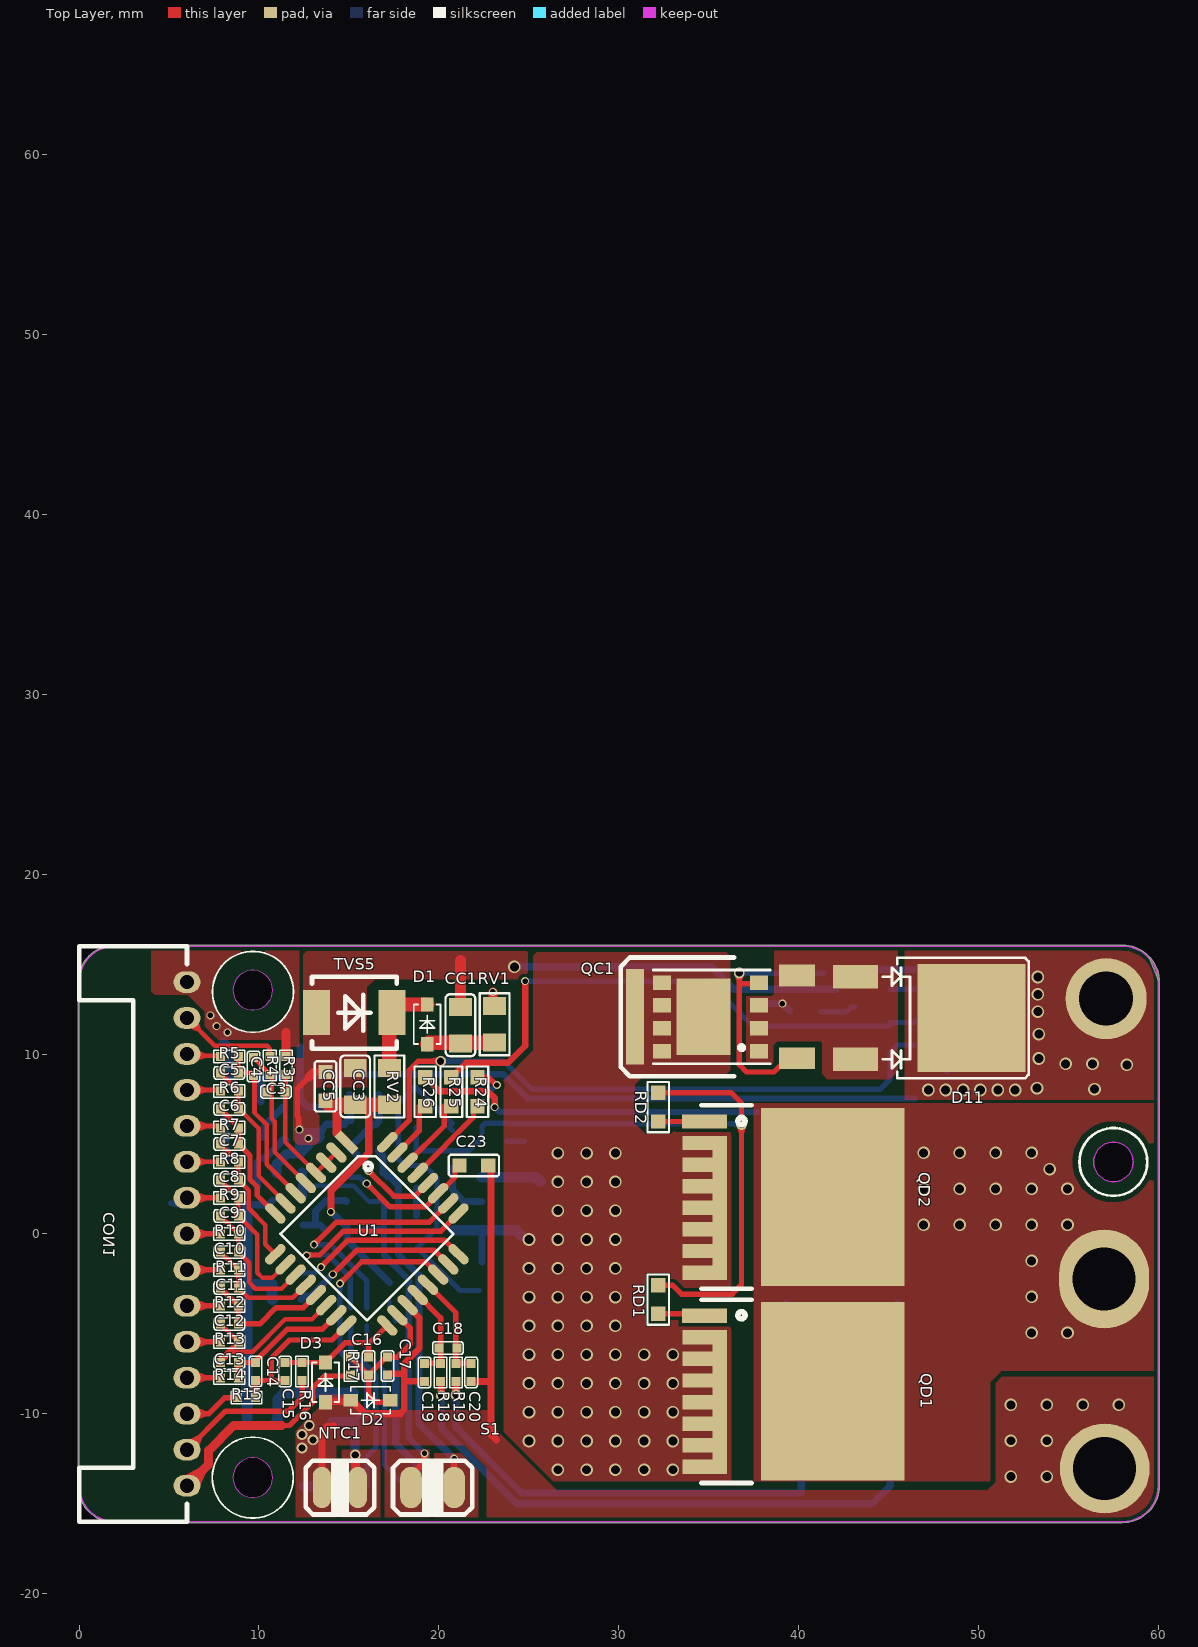
[diagram p0: Top Layer view]
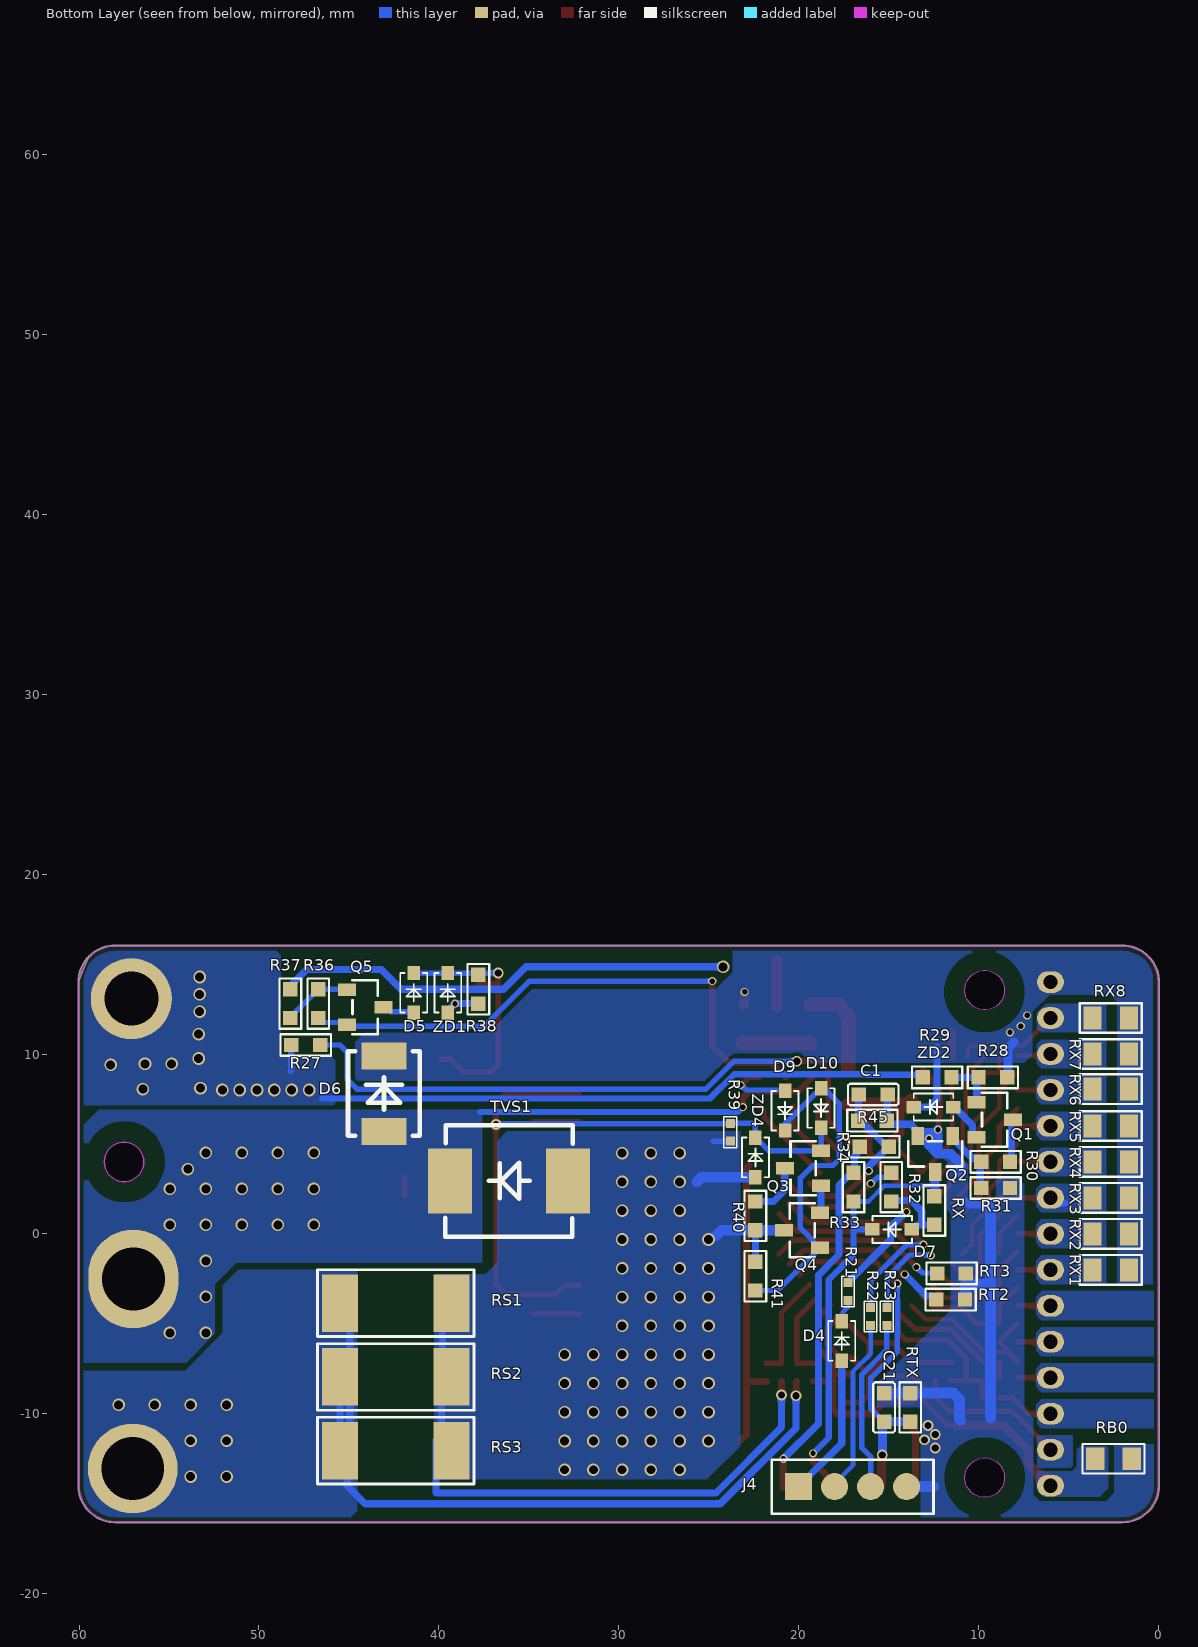
[diagram p1: Bottom Layer view, seen from below]
# Altium PCB MISC84412.PcbDoc
Units mm, origin at the board's own origin, x right, y up, seen from the top; angles counter-clockwise.
Board outline 60.1 x 32.1 mm, 2 copper layers (Top Layer, Bottom Layer); 110 components, 73 nets, 308 pads, 128 vias.

## Layer stack, top to bottom (the 12.6 mil dielectric is the usual default, probably not edited)
Top Solder: solder mask 0.0102, Solder Resist, Dk 3.5
Top Layer: signal copper 0.0356
Dielectric 1: dielectric 0.32, FR-4, Dk 4.8
Bottom Layer: signal copper 0.0356
Bottom Solder: solder mask 0.0102, Solder Resist, Dk 3.5

## Board outline
-0.05,-14.001 ccw(c2,-14) 2,-16.05 58,-16.05 ccw(c58,-14) 60.05,-14.001 60.05,14 60.05,-14 60.05,14 60.05,14.001 ccw(c58,14) 59.45,15.45 60.05,14.001 ccw(c58,14) 58,16.05 2,16.05 ccw(c2,14) -0.05,14
cut-out: 8.557,13.55 ccw(c9.657,13.55) 10.757,13.55 ccw(c9.657,13.55)
cut-out: 8.557,-13.55 ccw(c9.657,-13.55) 10.757,-13.55 ccw(c9.657,-13.55)
cut-out: 56.4,4 cw(c57.5,4) 58.6,4 cw(c57.5,4)

## Design rules (kind name [scope] priority, off if disabled: settings)
Clearance [All] p1: gap=0.2 ignorepadtopadclearanceinfootprint=FALSE
ComponentClearance [All] p1: gap=0 collisioncheckmode=3 verticalgap=0 showdistances=FALSE
HoleSize [All] p1: absolutevalues=TRUE maxlimit=50 minlimit=0.025 maxpercent=80.000 minpercent=20.000
HoleToHoleClearance [All] p1: gap=0 allowstackedmicrovias=TRUE
MinimumSolderMaskSliver [All] p1: minsoldermaskwidth=0
PlaneConnect [All] p1: planeconnectstyle=Direct reliefexpansion=0.508 reliefentries=4 reliefconductorwidth=0.254 reliefairgap=0.254
PolygonConnect [All] p1: connectstyle=Direct reliefconductorwidth=0.254 reliefentries=4 polygonreliefangle="90 Angle" airgapwidth=0.254
RoutingVias [All] p1: holewidth=0.4 width=0.6 viastyle="Through Hole" minholewidth=0.3 minwidth=0.45 maxholewidth=0.4 maxwidth=0.6
SilkToSilkClearance [All] p1: silktosilkclearance=0
SilkToSolderMaskClearance [IsPad] p1: minsilkscreentomaskgap=0 clearancetoexposedcopper=TRUE
SolderMaskExpansion [All] p1: expansion=0.102 istentingtop=FALSE
SupplyNets "Schematic Supply Nets_1" [InNet('B-')] p1: voltage=0.000
SupplyNets "Schematic Supply Nets" [InNet('VCC1')] p2: voltage=0.000
Width [All] p1: maxlimit=2 minlimit=0.254 preferedwidth=0.254 minimp=50.000000 maximp=50.000000 favimp=50.000000
23 further rules are at their usual default settings.

## Components (designator, comment, footprint, x,y, rotation, side; value= is the part's Value field where it differs from the comment)
C1 "0.1uF" C0603A 15.85,7.75 r180 bottom
C3 "0.1uF" C0402A 10.95,7.9 r0 top
C4 "0.1uF" C0402A 9.7,9.3 r90 top
C5 "0.1uF" C0402A 8.35,8.95 r0 top
C6 "0.1uF" C0402A 8.35,6.95 r0 top
C7 "0.1uF" C0402A 8.35,5 r0 top
C8 "0.1uF" C0402A 8.35,3 r0 top
C9 "0.1uF" C0402A 8.35,1 r0 top
C10 "0.1uF" C0402A 8.35,-1 r0 top
C11 "0.1uF" C0402A 8.35,-3 r0 top
C12 "0.1uF" C0402A 8.35,-5 r0 top
C13 "0.1uF" C0402A 8.35,-7.15 r180 top
C14 "0.1uF" C0402A 9.8,-7.65 r90 top
C15 "0.1uF" C0402A 11.45,-7.65 r270 top
C16 "0.1uF" C0402A 16.1,-7.35 r90 top
C17 "1uF" C0402A 17.15,-7.35 r90 top
C18 "1000PF" C0402A 20.5,-6.35 r180 top
C19 "1uF" C0402A 19.2,-7.7 r270 top
C20 "1uF" C0402A 21.8,-7.7 r270 top
C21 "1000PF" C0603A 15.25,-9.65 r90 bottom
C23 "1uF/25V" C0603A 21.95,3.8 r180 top
CC1 "1uF/100V" C0805L 21.2,11.6 r270 top
CC3 "1uF/100V" C0805L 15.35,8.2 r270 top
CC5 "100nF/100V" C0603A 13.7,8.2 r270 top
CON1 "Header 15" PH-2.0mm15P弯脚不带扣 6,0 r90 top locked
D1 "BAV21W" SOD323(1+2-) 19.35,11.65 r270 top
D2 "BAT46WS" SOD323(1+2-) 16.2,-9.25 r180 top
D3 "BAT46WS" SOD323(1+2-) 13.7,-8.25 r270 top
D4 "BAV21WS" SOD323(1+2-) 17.6,-5.95 r270 bottom
D5 "BAV21WS" SOD323(1+2-) 41.4,13.4 r270 bottom
D6 "RS3M" "SMB M(1+2-)" 43.05,7.8 r270 bottom
D7 "1N4148SW" SOD323 14.8,0.25 r180 bottom
D9 "BAV21WS" SOD323(1+2-) 20.75,6.85 r90 bottom
D10 "BAV21WS" SOD323(1+2-) 18.75,7 r90 bottom
D11 "MBR10100DCT" TO-252-DIODE-DUAL 46.387,12 r270 top
J4 "UART" CH-2.0-4P 17,-14.05 r180 bottom
NTC1 "10KNTC" RT2.3X1-2 14.5,-14.1 r180 top (schematic designator NC1)
Q1 "MMBT5401" SOT23-3_BEC 9.1,6.35 r270 bottom
Q2 "MMBT5551" SOT23-3_BEC 12.4,4.45 r0 bottom
Q3 "MMBT5401" SOT23-3 19.75,3.65 r90 bottom
Q4 "MMBT5401" SOT23-3 19.8,0.2 r90 bottom
Q5 "MMBT5401" SOT23-3 44.1,12.6 r270 bottom
QC1 "NMOS" TO-252-DFN 35.416,12.065 r0 top
QD1 "NMOS" TOLL 38.4,-8.75 r270 top value=60V75A@0.94
QD2 "NMOS" TOLL 38.4,2.05 r270 top value=60V75A@0.94
R3 "510R" R0402A 11.5,9.35 r90 top
R4 "510R" R0402A 10.6,9.35 r90 top
R5 "510R" R0402A 8.35,9.85 r180 top
R6 "510R" R0402A 8.35,7.95 r180 top
R7 "510R" R0402A 8.35,5.9 r180 top
R8 "510R" R0402A 8.35,4 r180 top
R9 "510R" R0402A 8.35,2 r180 top
R10 "510R" R0402A 8.35,0 r180 top
R11 "510R" R0402A 8.35,-2 r180 top
R12 "510R" R0402A 8.35,-4 r180 top
R13 "510R" R0402A 8.35,-6 r180 top
R14 "510R" R0402A 8.35,-8 r180 top
R15 "510R" R0402A 9.3,-9.1 r0 top
R16 "510R" R0402A 12.4,-7.65 r270 top
R17 "510R" R0402A 15.1,-7.35 r270 top
R18 "10R" R0402A 20.1,-7.7 r270 top
R19 "10R" R0402A 20.95,-7.7 r270 top
R21 "100R" R0402A 17.25,-3.2 r90 bottom
R22 "100R" R0402A 16,-4.6 r90 bottom
R23 "100R" R0402A 15.1,-4.6 r90 bottom
R24 "1K" R0603A#1 22.15,7.9 r270 top
R25 "1K" R0603A#1 20.7,7.9 r270 top
R26 "1M" R0603A#1 19.25,7.9 r270 top
R27 "3M" R0603A#2 47.4,10.5 r180 bottom
R28 "20K" R0603A#2 9.2,8.7 r180 bottom
R29 "100K" R0603A#2 12.3,8.7 r180 bottom
R30 "1M" R0603A#2 9.05,4 r180 bottom
R31 "100K" R0603A#2 9.05,2.55 r0 bottom
R32 "100K" R0603A#2 14.85,2.6 r270 bottom
R33 "0Ω/NC" R0603A#2 16.95,2.6 r270 bottom
R34 "100K" R0603A#2 15.8,4.85 r180 bottom
R36 "1M" R0603A#2 46.7,12.8 r270 bottom
R37 "3M" R0603A#2 48.25,12.8 r90 bottom
R38 "1M" R0603A#2 37.8,13.6 r90 bottom
R39 "10M" R0402A 23.8,5.65 r90 bottom
R40 "510R" R0603A#2 22.4,1 r270 bottom
R41 "4.7M" R0603A#2 22.4,-2.35 r270 bottom
R45 "10M" R0603A#2 15.9,6.3 r180 bottom
RB0 "51R" R0805L 2.5,-12.5 r0 bottom
RD1 "47R" R0603Ap 32.2,-3.65 r270 top
RD2 "47R" R0603Ap 32.2,7.05 r270 top
RS1 "R005" R2512L 42.4,-3.85 r180 bottom
RS2 "R005" R2512L 42.4,-7.95 r180 bottom
RS3 "R005" R2512L 42.4,-12.05 r180 bottom
RT2 "10K" R0603A#2 11.55,-3.65 r180 bottom
RT3 "10K" R0603A#2 11.5,-2.2 r180 bottom
RTX "NC" R0603A#2 13.8,-9.65 r90 bottom
RV1 "1KΩ" R0805L 23.1,11.65 r90 top
RV2 "100Ω" R0805L 17.25,8.2 r90 top
RX "0R" R0603A#2 12.45,1.3 r270 bottom
RX1 "0Ω" R0805L 2.65,-2 r0 bottom
RX2 "0Ω" R0805L 2.65,0 r0 bottom
RX3 "0Ω" R0805L 2.65,2 r0 bottom
RX4 "0Ω" R0805L 2.65,4 r0 bottom
RX5 "0Ω" R0805L 2.65,6 r0 bottom
RX6 "0Ω" R0805L 2.65,8.05 r0 bottom
RX7 "0Ω" R0805L 2.65,10 r0 bottom
RX8 "0Ω" R0805L 2.65,12 r0 bottom
S1 "SW-SPST" RT2.3X1.2-2 19.65,-14.1 r0 top
TVS1 "75CA" SMC 36.1,2.95 r0 bottom
TVS5 "SMBJ64A" "SMB M(1+2-)" 15.3,12.3 r180 top
U1 "SH3676016B" LQFP32L(PIN间距0.8mm) 16,0 r315 top
ZD1 "15V" SOD323(1+2-) 39.5,13.4 r270 bottom
ZD2 "15V" SOD323(1+2-) 12.5,7.05 r180 bottom
ZD4 "15V" SOD323(1+2-) 22.4,4.25 r270 bottom

## Footprints (in the part's own frame and the unit in brackets; to place one, negate y for a bottom-side part, rotate by r counter-clockwise, add the part's x,y. Pads: shape width x height; smd on the part's side, far side on the other; paste and mask are expansions set on the pad)
C0402A [mm] "贴片电容"
  rect 0.5x0.5 smd paste+0 mask+0.05: 1(-0.5,0) 2(0.5,0)
  silkscreen extent -0.85,-0.35 0.85,0.35
C0603A [mm] "贴片电容"
  rect 0.8x0.8 smd mask+0.08: 1(-0.8,0) 2(0.8,0)
  silkscreen extent -1.4,-0.6 1.4,0.6
C0805L [mil] "贴片电容"
  rect 40x50 smd paste+0 mask+1.97: 1(-40,0) 2(40,0)
  silkscreen extent -68,-32 68,32
CH-2.0-4P [mm] "测试座2.0mm"
  rect 1.5x1.5 smd: 1(-3,0)
  round 1.5 smd: 2(-1,0) 3(1,0) 4(3,0)
  silkscreen extent -4.5,-1.5 4.5,1.5
LQFP32L(PIN间距0.8mm) [mm] "贴片IC(中颖SH3676014/16BP)"
  rect 1.4x0.5 smd: 1(-4.4,2.8)
  oval 1.4x0.5 smd: 2(-4.4,2) 3(-4.4,1.2) 4(-4.4,0.4) 5(-4.4,-0.4) 6(-4.4,-1.2) 7(-4.4,-2) 8(-4.4,-2.8) 17(4.4,-2.8) 18(4.4,-2) 19(4.4,-1.2) 20(4.4,-0.4) 21(4.4,0.4) 22(4.4,1.2) 23(4.4,2) 24(4.4,2.8)
  oval 0.5x1.4 smd: 9(-2.8,-4.4) 10(-2,-4.4) 11(-1.2,-4.4) 12(-0.4,-4.4) 13(0.4,-4.4) 14(1.2,-4.4) 15(2,-4.4) 16(2.8,-4.4) 25(2.8,4.4) 26(2,4.4) 27(1.2,4.4) 28(0.4,4.4) 29(-0.4,4.4) 30(-1.2,4.4) 31(-2,4.4) 32(-2.8,4.4)
  silkscreen extent -3.4,-3.4 3.4,3.4
PH-2.0mm15P弯脚不带扣 [mm] "PH-2.0mm15P弯脚不带扣连接器"
  oval 1.2x1.5 hole 0.8: 1(-14,0) 2(-12,0) 3(-10,0) 4(-8,0) 5(-6,0) 6(-4,0) 7(-2,0) 8(0,0) 9(2,0) 10(4,0) 11(6,0) 12(8,0) 13(10,0) 14(12,0) 15(14,0)
  silkscreen extent -16,0 16,6
R0402A [mm] "贴片电阻"
  rect 0.5x0.5 smd paste+0 mask+0.05: 1(-0.5,0) 2(0.5,0)
  silkscreen extent -0.85,-0.35 0.85,0.35
R0603A#1 [mm] "贴片电阻"
  rect 0.8x0.8 smd mask+0.08: 1(-0.8,0) 2(0.8,0)
  silkscreen extent -1.4,-0.6 1.4,0.6
R0603A#2 [mm] "贴片电阻"
  rect 0.8x0.8 smd mask+0.102: 1(-0.8,0)
  rect 0.8x0.8 smd mask+0.08: 2(0.8,0)
  silkscreen extent -1.4,-0.6 1.4,0.6
R0603Ap [mm] "贴片电阻"
  rect 0.8x0.8 smd mask+0.08: 1(-0.8,0) 2(0.8,0)
  Top Layer pour cut-out: -1.5,0.7 1.5,0.7 1.5,-0.7 -1.5,-0.7
  silkscreen extent -1.4,-0.6 1.4,0.6
R0805L [mil] "贴片电阻"
  rect 40x50 smd paste+0 mask+1.97: 1(-40,0) 2(40,0)
  silkscreen extent -68,-32 68,32
R2512L [mm] "贴片电阻"
  rect 2x3.2 smd: 1(-3.1,0) 2(3.1,0)
  silkscreen extent -4.35,-1.85 4.35,1.85
RT2.3X1-2 [mm] "焊线NTC"
  oval 1x2.3 smd: 1(-1,0) 2(1,0)
  silkscreen extent -1.9,-1.55 1.9,1.5
RT2.3X1.2-2 [mm] "焊线NTC"
  oval 1.2x2.3 smd: 1(-1.2,0) 2(1.2,0)
  silkscreen extent -2.2,-1.55 2.2,1.5
"SMB M(1+2-)" [mm] "贴片二极管"
  rect 1.5x2.5 smd: 1(2.1,0) 2(-2.1,0)
  silkscreen extent -2.35,-2 2.35,2
SMC [mm]
  rect 2.44x3.62 smd: 1(-3.275,0) 2(3.275,0)
  silkscreen extent -3.55,-3.1 3.55,3.1
SOD323 [mm] "贴片二极管"
  rect 0.8x0.7 smd: 1(-1.1,0) 2(1.1,0)
  silkscreen extent -1.1,-0.75 1.1,0.75
SOD323(1+2-) [mm] "贴片二极管"
  rect 0.8x0.7 smd: 1(1.1,0) 2(-1.1,0)
  silkscreen extent -1.1,-0.75 1.1,0.75
SOT23-3 [mm] "贴片IC/MOS*"
  rect 0.7x1 smd: 1(-0.975,-1) 2(0.975,-1) 3(0,1.016)
  silkscreen extent -1.5,-0.7 1.5,0.7
SOT23-3_BEC [mm] "贴片IC/MOS*"
  rect 0.7x1 smd: B(-0.975,-1) C(0,1.016) E(0.975,-1)
  silkscreen extent -1.5,-0.7 1.5,0.7
TO-252-DFN [mm]
  rect 1x0.8 smd: 1(2.384,1.905) 2(2.384,-1.905) 2(2.384,-0.635) 2(2.384,0.635) 3(-3.016,-1.905) 3(-3.016,-0.635) 3(-3.016,0.635) 3(-3.016,1.905)
  rect 2x1.2 smd: 1(4.5,-2.3) 2(4.5,2.3)
  rect 1x5.3 smd: 3(-4.5,0)
  rect 3x4.26 smd: 3(-0.716,0)
  silkscreen extent -5.31,-3.3 3,3.3
TO-252-DIODE-DUAL [mm] "贴片二极管"
  rect 1.3x2.5 smd: 1(-2.3,-3.212) 2(2.3,-3.212)
  rect 6x6 smd: 3(0,3.213)
  silkscreen extent -3.35,-1.7 3.35,6.4
TOLL [mm] "贴片MOS"
  rect 0.8x2.5 smd: 1(-4.2,-3.638)
  rect 0.8x1.7 smd: 2(-3,-4) 2(-1.8,-4) 2(-0.6,-4) 2(0.6,-4) 2(1.8,-4) 2(3,-4) 2(4.2,-4)
  rect 8x0.8 smd: 2(0.6,-2.788)
  rect 9.9x8 smd: 3(0,3.5)
  silkscreen extent -5.1,-3.8 5.1,-1

## Part data
C1 C23: library part CAP, "CAP"
C3 C4 C5 C6 C7 C8 C9 C10 C11 C12 C13 C14 C15 C16 C17 C18 C19 C20 C21 CC1 CC3 CC5: library part "0805 100nF(104) 10% 50V", "SMD capacitor", Package=0805, SuppliersPartNumber=C49678
CON1: "Header15"
D1: library part "SOD-323 1N4148WS T4", "Diode", Package=SOD-323, SuppliersPartNumber=C2128
D2 D3 D4 D5 D6 D9 D10: library part DIODE, "DIODE"
D7: "SMD diode"
D11: "SMD dual diode, common cathode"
J4: library part CON4
NTC1 RT2 RT3: library part RES2, "RES"
Q1: library part PNP, "PNP Transistor"
Q2: library part NPN, "NPN Transistor"
Q3 Q4 Q5: library part 8550, "PNP"
QC1: library part MOSFET-N
QD1 QD2: library part IRFR014, "HEXFET N-Channel Power MOSFET"
R3 R4 R5 R6 R7 R8 R9 R10 R11 R12 R13 R14 R15 R16 R17 R18 R19 RS1 RS2 RS3: library part "0603 1KΩ (1001) 1%", "SMD resistor", Package=0603, SuppliersPartNumber=C21190
R21 R22 R23 R24 R25 R26 R27 R28 R29 R30 R31 R32 R33 R34 R36 R37 R38 R39 R40 R41 R45 RTX RX: library part RES1, "RES"
RB0: library part RES1, "±5% /UniOhm/yageo/TA-I/Walsin/Ralec"
RD1 RD2: library part "0603 1.2MΩ (1204) 1%", "SMD resistor", Package=0603, SuppliersPartNumber=C22766
RV1 RV2 RX1 RX2 RX3 RX4 RX5 RX6 RX7 RX8: library part "0805 300Ω (3000) 1%", "SMD resistor", Package=0805, SuppliersPartNumber=C17617
S1: "Single-Pole, Single-Throw Switch"
TVS1: library part TVS, "TVS"
TVS5: library part "LL-34 ZMM5V6", "Zener diode", Package=LL-34, SuppliersPartNumber=C8062
ZD1 ZD2 ZD4: library part ZENOR, "ZENOR"

## Free pads (board coordinates)
  round 0.025 on Keep-Out: 1(52.327,65.458) 1(56.137,-19.886)
  rect 2.5x15 on Bottom Solder: 2(25.9,-3.65) 2(29.039,-3.638)
  rect 2.5x15 on Top Solder: 2(26.3,-4.85) 2(29.3,-4.85)
  rect 2.5x20 on Top Solder: 2(48.7,-3.35)
  rect 2.5x12 on Top Solder: 2(51.789,0.262)
  oval 5x5.5 hole 3.5: 2(56.986,-2.51)
  round 5 hole 3.5: 2(57.017,-13.049)
  round 4.5 hole 3: 2(57.098,13.075)

## Via types
v1: diameter 0.7, hole 0.5, Top Layer to Bottom Layer, tented both sides, 98 vias
v2: diameter 0.45, hole 0.3, Top Layer to Bottom Layer, tented both sides, 20 vias
v3: diameter 0.6, hole 0.4, Top Layer to Bottom Layer, tented both sides, 10 vias

## Nets (pads, with @x,y where several pads share a name; then routed paths per layer and width w, separated by ;. In a path a pad name is that pad's centre, name@x,y a point inside that pad or via, vN(x,y) a via of type N, cw(c..) or ccw(c..) an arc to the next point about the centre after c; other vN are vias at no path point)
B0: CON1.1 R17.2 RB0.2 | length 12.6
  Top Layer w0.3: 11.25,-10.65 11.7,-10.65 12.55,-9.8 13,-9.35 13,-8.55 13.65,-7.9 15.1,-7.9 R17.2
  Top Layer w0.5: CON1.1 7.2,-12.8 7.2,-12.05 8.6,-10.65 11.25,-10.65
B1: CON1.2 R16.2 | length 8.6
  Top Layer w0.3: CON1.2 8.15,-9.85 11.65,-9.85 12.4,-9.1 R16.2
B2: CON1.3 R15.1 | length 3.2
  Top Layer w0.3: CON1.3 7.2,-10 8.1,-9.1 R15.1
B3: CON1.4 R14.2 | length 1.9
  Top Layer w0.3: CON1.4 R14.2
B4: CON1.5 R13.2 | length 2
  Top Layer w0.3: CON1.5@6.1,-5.9 CON1.5 R13.2
B5: CON1.6 R12.2 | length 2.1
  Top Layer w0.3: CON1.6@6.2,-4.2 CON1.6 R12.2
B6: CON1.7 R11.2 RX1.2 | length 1.9
  Top Layer w0.3: CON1.7 R11.2
B7: CON1.8 R10.2 RX2.2 | length 1.9
  Top Layer w0.3: CON1.8 R10.2
B8: CON1.9 R9.2 RX3.2 | length 2.8
  Top Layer w0.3: CON1.9 R9.2@7.8,2
  Bottom Layer w0.3: 5.1,1.7 CON1.9@6,1.7 ; CON1.9 CON1.9@6.1,1.9
B9: CON1.10 R8.2 RX4.2 | length 1.9
  Top Layer w0.254: CON1.10 R8.2
B10: CON1.11 R7.2 RX5.2 | length 1.9
  Top Layer w0.3: CON1.11 R7.2@7.85,6
B11: CON1.12 R6.2 RX6.2 | length 2.3
  Top Layer w0.254: CON1.12@6.34,7.66 CON1.12 R6.2@7.85,8
B12: CON1.13 R5.2 RX7.2 | length 1.9
  Top Layer w0.254: CON1.13 6.1,9.9 R5.2@7.85,9.9
B13: CON1.14 R4.2 RX8.2 | length 5.8
  Top Layer w0.254: CON1.14 7.55,10.45 10.451,10.45 10.6,10.301 R4.2
B+: CON1.15 D6.2 R3.2 R28.2 RV1.2 RX1.1 RX2.1 RX3.1 RX4.1 RX5.1 RX6.1 RX7.1 RX8.1 ZD2.2 | length 8.8
  Top Layer w0.5: R3.2 11.5,11.191 ; v2(23,13.45) 23,12.766 RV1.2
  Bottom Layer w0.4: 12.3,10.375 12.3,7.484 12.734,7.05 ZD2.2
  Bottom Layer w0.5: 8.035,10.665 8.35,10.35 R28.2@8.35,8.55
  other v2: 8.25,11.2 7.65,11.55 7.3,12.15
B-: C1.2 C17.1 C19.2 C20.2 C21.2 C23.1 CC1.1 CC3.1 CC5.1 D2.1 D3.1 J4.4 NTC1.2 pad.2@57.017,-13.049 Q2.E R18.2 R31.1 R37.2 R45.2 RB0.1 RS1.1 RS2.1 RS3.1 RT2.2 RT3.2 RTX.2 TVS5.1 U1.19 | length 143.1
  Top Layer w0.3: v2(12.25,5.8) 12.221,5.829 12.221,6.459 12.125,6.555 12.125,8.06 12.791,8.726
  Top Layer w0.35: C17.1 17.225,-7.775 18.05,-7.775 18.075,-7.8 18.075,-8.1 ; 17.866,-10 17.916,-9.95 17.916,-9.915 18.075,-9.755 18.075,-8.1 ; 18.075,-7.775 18.075,-7.204 18.925,-6.354 18.925,-4.663 18.263,-4 U1.19 ; C19.2 18.175,-8.2 18.075,-8.1 ; R18.2 20.125,-8.225 v3@20.125,-8.975
  Top Layer w0.4: 13.075,9.01 13.1,9.01 ; NTC1.2 13.5,-11 13.812,-10.688 14.112,-10.688 14.15,-10.65 ; D3.1 13.75,-9.3 D2.1@15.1,-9.3 ; D2.1 15.15,-9.25 15.9,-10 17.866,-10 ; C20.2 22.85,-8.2 22.9,-8.15 ; C23.1 22.9,3.65 22.9,-8.15 ; 23.2,-11.45 22.9,-11.15 22.9,-8.15
  Top Layer w0.5: 12.791,8.726 13.075,9.01
  Top Layer w0.6: CC1.1 21.2,15.2
  Bottom Layer w0.4: 9.331,1.469 9.331,1.619 10.516,1.619 10.75,1.853 ; v2(12.25,5.8) 12.267,5.783 12.434,5.616 v2@12.6,5.45 ; Q2.E@13.362,5.713 13.487,5.713 13.525,5.75 13.525,5.862 13.759,6.096 14.746,6.096 R45.2@14.95,6.3 ; C1.2 15.075,7.725 15.075,6.325 R45.2 ; v3(20.15,-9) 20.15,-10.8 24.35,-15 44.112,-15 45.097,-14.016 45.097,-12.653 RS3.1@45.5,-12.25 ; v1(24.2,14.85) 35.15,14.85 36.4,13.6 42.1,13.6 43.2,14.7 47.35,14.7 R37.2@48.25,13.8 ; RS2.1@45.5,-8.05 RS3.1 RS3.1@45.5,-12.25 ; RS1.1 44.95,-4.4 44.95,-7.95 44.95,-12.25 RS3.1@45.5,-12.25
  Bottom Layer w0.55: 10.966,3.389 10.966,3.871 11.548,4.452 12.267,4.452 ; v2@12.267,5.783 12.267,4.452 ; 12.434,5.616 13.3,5.616 13.375,5.541 Q2.E 13.375,5.375 13.3,5.3 v2(12.75,5.3) 12.75,4.935 12.267,4.452
  Bottom Layer w0.6: 9.331,-10.237 9.331,1.469 ; 9.406,-2.8 10.725,-2.8 10.725,-3.625 RT2.2 ; 11,-10.35 11.05,-10.3 11.05,-9.201 11.401,-8.85 RTX.2 C21.2 ; 12.5,-14.05 J4.4 ; C21.2@15.244,-8.844 C21.2@15.25,-8.837
  other v1: 51.8,-13.5 53.8,-13.5 51.8,-11.5 53.8,-11.5 51.8,-9.5 53.8,-9.5 55.8,-9.5 57.8,-9.5
  other v3: 12.4,-11.9 13,-11.45 12.4,-11.15 12.8,-10.65
C-: D11.3 pad.2@57.098,13.075 R27.1 R29.1 | length 35.5
  Bottom Layer w0.35: R29.1 13.25,8.85 16.2,8.85 16.225,8.875 23.583,8.875 24.933,7.525 46.475,7.525 ; R27.1 48.2,9.1 48.25,9.05
  other v1: 47.214,8 48.179,8 49.143,8 50.107,8 51.071,8 52.036,8 56.45,8.05 53.25,8.1 58.25,9.4 54.85,9.45 56.336,9.45 53.35,9.75 53.35,11.1 53.3,12.35 53.3,13.314 53.3,14.279
CHG1: Q5.2 R25.1 R36.2 | length 31.5
  Top Layer w0.35: R25.1 21.512,9.513 23.862,9.513 24.8,10.45 v2(24.8,14.05)
  Bottom Layer w0.3: v2(24.8,14.05) 34.95,14.05 37.45,11.55 45.025,11.55 Q5.2 ; Q5.2@45.1,11.75 46.45,11.75 R36.2
CTLD: C1.1 R34.2 R45.1 U1.28 | length 9.4
  Top Layer w0.3: v2(16.1,3.5) 17.5,2.1 18.666,2.1 U1.28
  Bottom Layer w0.4: R34.2 16.09,3.76 16.09,3.51 v2(16.1,3.5) ; R34.2@15.25,5 16.35,6.1 16.5,6.1 16.675,6.275 16.675,7.725 C1.1
DSG1: D9.1 R24.1 | length 3.9
  Top Layer w0.3: R24.1 22.759,8.7 23.184,8.275 v2(23.225,8.275)
  Bottom Layer w0.3: D9.1 20.8,8 22.909,8 23.184,8.275 v2(23.225,8.275)
NetC18_1: C18.1 C20.1 R19.1 U1.21 | length 5.9
  Top Layer w0.3: U1.21 20.95,-4.384 R19.1 C20.1
NetC18_2: C18.2 C19.1 R18.1 U1.20 | length 5.2
  Top Layer w0.3: U1.20 20.1,-4.666 R18.1 C19.1
NetC21_1: C21.1 NTC1.1 RTX.1 U1.22 | length 19.8
  Top Layer w0.3: v2(14.507,-2.757) 15.714,-1.55 19.247,-1.55 U1.22
  Top Layer w0.5: v3(15.35,-12.3) 15.369,-12.319 15.369,-12.966 15.404,-13.001 15.404,-14.004 NTC1.1
  Bottom Layer w0.3: v2(14.507,-2.757) 14.507,-3.698 14.5,-3.705 14.5,-5.495 14.507,-5.502 14.507,-6.551 16,-8.044 16,-9.7 15.331,-10.369 C21.1@15.331,-10.6
  Bottom Layer w0.5: RTX.1@14.05,-10.45 14.063,-10.438 C21.1@15.25,-10.438 ; C21.1@15.331,-10.6 15.331,-12.281 v3(15.35,-12.3)
NetCC1_2: CC1.2 D1.1 RV1.1 | length 3.8
  Top Layer w0.8: D1.1 19.434,10.634 RV1.1
NetD1_2: D1.2 RV2.2 TVS5.2 | length 4.9
  Top Layer w0.8: RV2.2@17.25,9.108 17.25,12.15 TVS5.2 ; TVS5.2@17.75,12.75 D1.2
NetD4_1: D4.1 J4.1 | length 8
  Bottom Layer w0.4: D4.1 17.6,-11.65 J4.1
NetD4_2: D4.2 R21.1 | length 1.3
  Bottom Layer w0.254: R21.1 17.25,-4.05 17.55,-4.35 17.55,-4.8 D4.2
NetD5_1: D5.1 Q5.3 | length 1.9
  Bottom Layer w0.3: D5.1@41.25,12.35 42.684,12.35 42.934,12.6 Q5.3
NetD5_2: D5.2 QC1.1 R38.2 ZD1.2 | length 14.6
  Top Layer w0.3: v3(36.7,14.5) 36.7,13.9 ; QC1.1@37.8,13.905 36.705,13.905 36.7,13.9 ; QC1.1@39.916,9.7 39.327,9.7 38.627,9 37.104,9 36.7,9.404 36.7,13.9
  Bottom Layer w0.3: v3(36.7,14.5) R38.2@37.8,14.5 ; R38.2 37.9,14.5 ZD1.2 D5.2
NetD7_1: D7.1 Q2.C R33.2 RX.1 S1.1 | length 24.4
  Top Layer w0.35: S1.1 18.45,-13.421 19.181,-12.69 19.181,-12.219 v2(19.2,-12.2)
  Bottom Layer w0.254: 12.425,2.7 12.452,2.673 15.239,2.673 16.112,1.8 R33.2
  Bottom Layer w0.35: D7.1 16.85,0.25 16.95,0.15 ; R33.2@16.95,1.75 16.95,0.15 ; v2@19.187,-12.187 18.325,-11.325 18.325,-2.55 16.95,-1.175 16.95,0.15
  Bottom Layer w0.5: Q2.C 12.425,3.409 12.425,2.7 12.425,2.125 RX.1
NetD7_2: D7.2 R32.2 RX.2 | length 4.1
  Bottom Layer w0.4: RX.2 13.05,0.5 ; D7.2 13.65,0.25 13.4,0.5 13.05,0.5 ; R32.2 14.8,1.85 13.741,1.85 13.15,1.259 13.15,0.6 13.05,0.5
NetD9_2: D9.2 D10.1 Q4.1 R41.2 | length 18.8
  Bottom Layer w0.3: D10.1@18.675,8.175 17.75,7.25 17.75,4.15 18.1,3.8 19.2,3.8 19.9,3.1 19.9,0.325 Q4.1 21.175,-3.15 R41.2@22.25,-3.15 ; D10.1 20.557,6.293 20.7,6.15 20.75,6.15 ; D9.2@20.582,5.918 D9.2
NetD10_2: D10.2 Q3.2 R39.2 RD1.1 RD2.1 ZD4.2 | length 40.4
  Top Layer w0.3: RD1.1 33,-2.85 33.5,-3.35 36.3,-3.35 36.825,-2.825 v3(36.825,6.075) 36.825,7.275 36.25,7.85 RD2.1
  Bottom Layer w0.3: D10.2 Q3.2 21.675,4.625 22.15,5.1 22.2,5.1 22.4,5.3 ZD4.2 22.4,5.974 22.576,6.15 R39.2 23.838,6.112 31.917,6.112 36.788,6.112 v3(36.825,6.075)
NetD11_1: D11.1 D11.2 QC1.2 R38.1 ZD1.1 | length 1.9
  Bottom Layer w0.4: R38.1 v2(39.1,12.8) ZD1.1@39.5,12.4
NetJ4_2: J4.2 R22.1 | length 9.8
  Bottom Layer w0.254: R22.1 16,-6.662 16.977,-7.639 16.977,-12.855 18,-13.878 J4.2
NetJ4_3: J4.3 R23.1 | length 9.7
  Bottom Layer w0.3: R23.1 15.1,-6.437 16.5,-7.837 16.5,-11.888 16,-12.388 J4.3
NetQ1_B: Q1.B R28.1 R29.2 | length 2.8
  Bottom Layer w0.4: R28.1 R29.2 ; Q1.B R28.1@10.1,8.65
NetQ1_C: Q1.C R30.2 | length 2.4
  Bottom Layer w0.4: Q1.C 8.167,6.267 8.167,4.083 R30.2
NetQ1_E: Q1.E ZD2.1 | length 2.3
  Bottom Layer w0.4: Q1.E 10.187,5.375 10.337,5.525 10.337,6.037 11.35,7.05 ZD2.1
NetQ2_B: Q2.B R30.1 R31.2 | length 3.2
  Bottom Layer w0.4: R31.2@9.9,2.65 9.9,3.55 9.9,3.75 R30.1@9.9,3.95 ; R30.1@10.05,4.2 10.341,4.2 11,4.859 11,4.875 11.325,5.2 Q2.B@11.5,5.2
NetQ3_1: Q3.1 Q4.2 | length 1.5
  Bottom Layer w0.4: Q4.2@18.75,1.025 Q3.1@18.75,2.535
NetQ3_3: Q3.3 R40.1 | length 3.1
  Bottom Layer w0.4: Q3.3 20.766,2.434 21.4,1.8 R40.1
NetQ5_1: Q5.1 R36.1 R37.1 | length 3.9
  Bottom Layer w0.3: Q5.1 45.125,13.6 R36.1 48,12.3 48,12.25 R37.1
NetQD1_1: QD1.1 RD1.2 | length 2.6
  Top Layer w0.3: RD1.2 QD1.1@34.762,-4.45
NetQD2_1: QD2.1 RD2.2 | length 2.6
  Top Layer w0.3: RD2.2 QD2.1
NetR24_2: R24.2 U1.29 | length 5.1
  Top Layer w0.3: U1.29 21.924,6.49 21.924,6.874 R24.2
NetR25_2: R25.2 U1.30 | length 4
  Top Layer w0.3: U1.30 20.3,5.997 R25.2@20.3,7.1
NetR26_2: R26.2 U1.31 | length 3.1
  Top Layer w0.3: U1.31 18.9,5.728 R26.2@18.9,7.1
NetR27_2: R27.2 U1.32 | length 35.5
  Top Layer w0.3: U1.32 17.136,5.091 18.35,6.305 18.35,9.095 18.855,9.6 v3(20.1,9.6)
  Bottom Layer w0.3: v3(20.1,9.6) 23.6,9.6 25.15,8.05 44.55,8.05 45.1,8.6 45.1,10.113 45.487,10.5 R27.2
NetR33_1: R33.1 R34.1 S1.2 | length 20.5
  Top Layer w0.4: S1.2 v2(20.85,-12.5)
  Bottom Layer w0.4: R34.1@16.65,4.6 16.9,4.35 16.9,3.4 16.95,3.35 17,3.35 17.15,3.2 17.25,3.2 17.75,2.7 17.75,-1.15 18.9,-2.3 18.9,-10.55 v2(20.85,-12.5)
NetRT2_1: RT2.1 U1.23 | length 9.6
  Top Layer w0.3: v2(14.1,-2.25) 15.45,-0.9 19.728,-0.9 U1.23
  Bottom Layer w0.4: RT2.1 12.55,-3.45 12.9,-3.45 v2@14.09,-2.26
NetRT3_1: RT3.1 U1.24 | length 9.9
  Top Layer w0.3: v2(13.45,-1.85) 14.95,-0.35 20.31,-0.35 U1.24
  Bottom Layer w0.3: RT3.1 12.325,-2.175 13.125,-2.175 v2(13.45,-1.85)
P-: D6.1 pad.2@56.986,-2.51 QD1.3 QD2.3 R26.1 TVS1.2 | length 20.5
  Top Layer w0.35: R26.1 20.025,7.925 22.726,7.925 23.1,7.551 v2(23.1,7.05) ; QD2.3@41.9,2.15 QD2.3@41.9,3.1
  Bottom Layer w0.35: v2(23.1,7.05) 23.375,6.775 37.7,6.775
  other v1: 52.95,-5.5 54.95,-5.5 52.95,-3.5 52.95,-1.5 46.95,0.5 48.95,0.5 50.95,0.5 52.95,0.5 54.95,0.5 46.95,2.5 48.95,2.5 50.95,2.5 52.95,2.5 54.95,2.5 53.95,3.6 46.95,4.5 48.95,4.5 50.95,4.5 52.95,4.5
RS2: Q4.3 QC1.3 QD1.2 QD2.2 R19.2 R39.1 R40.2 R41.1 RS1.2 RS2.2 RS3.2 TVS1.1 ZD4.1 | length 46.1
  Top Layer w0.4: v3(20.95,-8.95) R19.2
  Bottom Layer w0.3: R39.1 24.75,5.15
  Bottom Layer w0.4: v3(20.95,-8.95) 20.95,-10.75 24.6,-14.4 40.15,-14.4 40.15,-11.6 RS3.2@40.15,-11.45 ; R41.1 R40.2 ; RS3.2 39.85,-11.5 39.85,-8.6 RS2.2@39.3,-8.05 ; RS2.2 39.8,-7.45 39.8,-4.35 RS1.2 ; RS3.2@39.4,-12.15 39.95,-11.6 RS3.2@40.1,-11.45
  Bottom Layer w0.6: Q4.3 24.3,0.2 24.6,-0.1 ; ZD4.1 25.4,3.15 25.65,2.9
  other v1: 26.611,-13.112 28.211,-13.112 29.811,-13.112 31.411,-13.112 33.011,-13.112 25.011,-11.512 26.611,-11.512 28.211,-11.512 29.811,-11.512 31.411,-11.512 33.011,-11.512 25.011,-9.912 26.611,-9.912 28.211,-9.912 29.811,-9.912 31.411,-9.912 33.011,-9.912 25.011,-8.312 26.611,-8.312 28.211,-8.312 29.811,-8.312 31.411,-8.312 33.011,-8.312 25.011,-6.712 26.611,-6.712 28.211,-6.712 29.811,-6.712 31.411,-6.712 33.011,-6.712 25.011,-5.112 26.611,-5.112 28.211,-5.112 29.811,-5.112 25.011,-3.512 26.611,-3.512 28.211,-3.512 29.811,-3.512 25.011,-1.912 26.611,-1.912 28.211,-1.912 29.811,-1.912 25.011,-0.312 26.611,-0.312 28.211,-0.312 29.811,-0.312 26.611,1.288 28.211,1.288 29.811,1.288 26.611,2.888 28.211,2.888 29.811,2.888 26.611,4.488 28.211,4.488 29.811,4.488
RXD1: R23.2 U1.25 | length 14.1
  Top Layer w0.3: v2(12.65,-1.2) 12.679,-1.171 13.379,-1.171 14.7,0.15 20.11,0.15 U1.25
  Bottom Layer w0.3: v2(12.65,-1.2) 12.679,-1.171 13.834,-1.171 15.082,-2.419 15.082,-3.255 15.073,-3.264 15.073,-4.073 R23.2
TXD1: R22.2 U1.26 | length 13.7
  Top Layer w0.3: v2(13.057,-0.596) 14.303,0.65 19.478,0.65 U1.26
  Bottom Layer w0.3: v2(13.057,-0.596) 13.967,-0.596 16,-2.63 R22.2
VBAT1: CC3.2 CC5.2 R21.2 RV2.1 U1.1 | length 18.2
  Top Layer w0.4: v2(14,1.225) 14,2.4 16.1,4.5 16.1,7.184
  Top Layer w0.5: CC3.2@14.773,7.184 14.35,6.761 14.35,5.61 U1.1
  Top Layer w0.8: CC5.2 13.916,7.184 14.773,7.184 16.1,7.184 RV2.1
  Bottom Layer w0.4: v2(14,1.225) 14.014,1.225 14.239,1 14.266,1 14.9,0.366 14.9,-0.35 R21.2
VC0: C16.1 C17.2 D2.2 R17.1 U1.18 | length 8.8
  Top Layer w0.3: R17.1 C16.1 ; D2.2@17.35,-9.35 16.5,-9.35 16.1,-8.95 C16.1 ; U1.18 18.4,-5.228 18.4,-6.136 17.686,-6.85 C17.2 17.1,-6.85 C16.1
VC1: C15.1 C16.2 D3.2 R16.1 U1.17 | length 7.4
  Top Layer w0.3: C15.1 R16.1 D3.2 14.8,-6.05 16.173,-6.05 ; C16.2 16.1,-6.123 16.173,-6.05 ; U1.17 16.173,-6.05
VC2: C14.1 C15.2 R15.2 U1.16 | length 8.9
  Top Layer w0.3: R15.2 C14.1 10.675,-8.15 ; C15.2@11.55,-8.15 10.675,-8.15 ; U1.16 14.06,-5.9 11.7,-5.9 10.675,-6.925 10.675,-8.15
VC3: C13.1 C14.2 R14.1 U1.15 | length 7.4
  Top Layer w0.3: R14.1 C13.1 9.725,-7.15 11.575,-5.3 13.528,-5.3 U1.15
VC4: C12.1 C13.2 R13.1 U1.14 | length 10.2
  Top Layer w0.254: C12.1 R13.1 8.375,-6.475 7.85,-7 C13.2 7.925,-7.075 8.45,-6.55 9.65,-6.55 11.45,-4.75 12.947,-4.75 U1.14
VC5: C11.1 C12.2 R12.1 U1.13 | length 7.4
  Top Layer w0.3: C11.1 R12.1 C12.2 10.05,-5 10.95,-4.1 12.466,-4.1 U1.13
VC6: C10.1 C11.2 R11.1 U1.12 | length 6.7
  Top Layer w0.254: C10.1 R11.1 C11.2 9.4,-3.55 11.884,-3.55 U1.12
VC7: C9.1 C10.2 R10.1 U1.11 | length 7.4
  Top Layer w0.254: C9.1 R10.1 C10.2 9.45,-1.6 9.45,-2.7 9.8,-3.05 11.253,-3.05 U1.11
VC8: C8.1 C9.2 R9.1 U1.10 | length 8
  Top Layer w0.254: C8.1 R9.1 C9.2@8.85,1.05 ; C9.2 9.9,-0.05 9.9,-0.349 9.904,-0.353 9.904,-2.154 10.2,-2.45 10.722,-2.45 U1.10
VC9: C7.1 C8.2 R8.1 U1.9 | length 7.4
  Top Layer w0.254: C7.1 R8.1 C8.2 9.427,2.423 9.427,1.423 10.358,0.492 10.358,-0.581 U1.9
VC10: C6.1 C7.2 R7.1 U1.8 | length 7.1
  Top Layer w0.3: C6.1 8.75,6.05 8.75,6 8.85,6 R7.1 C7.2 9.5,4.35 9.5,3.025 9.904,2.621 9.904,2.136 U1.8
VC11: C5.1 C6.2 R6.1 U1.7 | length 8.7
  Top Layer w0.254: C5.1 R6.1 ; R6.1@8.85,7.9 8.85,7 9.977,5.873 9.977,3.222 11.475,1.725 U1.7
VC12: C4.1 C5.2 R5.1 U1.6 | length 9.3
  Top Layer w0.254: R5.1@8.85,9.8 C5.2 9.6,8.95 9.75,8.8 9.75,6.742 10.431,6.061 10.431,3.872 U1.6
VC13: C3.1 C4.2 R4.1 U1.5 | length 8.2
  Top Layer w0.254: C4.2@9.7,9.788 9.712,9.788 9.823,9.677 9.823,9.665 10.7,8.788 10.7,6.434 10.885,6.249 10.885,4.549 U1.5
VC14: C3.2 R3.1 U1.2 U1.3 U1.4 | length 7.7
  Top Layer w0.254: C3.2 11.45,5.116 U1.4 U1.3 U1.2 ; C3.2@11.5,7.9 R3.1@11.5,8.75
VCC1: C23.2 R32.1 U1.27 | length 8.3
  Top Layer w0.3: v2(15.992,2.794) 17.287,1.5 19.251,1.5 20.9,3.149 20.9,3.55 C23.2
  Bottom Layer w0.3: R32.1 15.1,3.15 15.596,3.15 15.952,2.794 v2(15.992,2.794)

## Polygon pours and split planes (outlines as drawn)
B+ on Bottom Layer "NONET_L-01_P-001" (solid, remove dead copper, pour order 0): 19.3,9.5 19.85,10.05 23.6,10.05 25.15,8.5 44.6,8.5 44.65,8.55 44.65,10.65 44.1,11.2 37.2,11.2 34.8,13.6 29.625,13.6 24.6,13.6 23.65,14.55 23.65,15.9 1.4,15.9 0.3,14.8 0.3,-2.8 2.3,-2.8 2.3,12.9 2.7,13.3 6.05,13.3 7,12.35 7,9.95 7.45,9.5
RS2 on Bottom Layer "RS2_L02_P042" (solid, remove dead copper, pour order 42): 37.4,-2.25 36.75,-1.6 36.75,5.162 36.212,5.7 23.25,5.7 23.25,-11.8 25.1,-13.65 40.25,-13.65 40.25,-2.3 40.2,-2.25
P- on Bottom Layer "P-_L02_P041" (solid, remove dead copper, pour order 41): 37.6,-1.6 37.6,6.9 58.9,6.9 59.9,5.9 59.9,-7.15 54.05,-7.15 52.45,-5.55 52.45,-2.8 51.25,-1.6
B- on Bottom Layer "NONET_L-01_P-001" (solid, pour order 17): 54.1,-7.6 52,-5.5 52,-2.85 51.15,-2 44.55,-2 44.55,-15.4 45.15,-16 58.8,-16 60,-14.8 60,-7.6
B0 on Bottom Layer "NONET_L-01_P-001" (solid, pour order 21): 2.9,-11.8 2.8,-11.9 2.8,-14.15 3.25,-14.6 6.4,-14.6 6.75,-14.25 6.75,-13.2 4.8,-13.2 4.55,-12.95 4.55,-12 4.35,-11.8
B1 on Bottom Layer "NONET_L-01_P-001" (solid, remove dead copper, pour order 49): 4.75,-12.862 4.884,-13 6.8,-13 6.8,-11.2 5.3,-11.2 4.75,-11.2
B2 on Bottom Layer "NONET_L-01_P-001" (solid, remove dead copper, pour order 48): -0.05,-9.2 -0.05,-10.8 6.5,-10.8 6.777,-10.523 6.777,-9.477 6.5,-9.2
B3 on Bottom Layer "NONET_L-01_P-001" (solid, remove dead copper, pour order 47): -0.05,-7.2 -0.05,-8.8 6.5,-8.8 6.8,-8.5 6.8,-7.5 6.5,-7.2
B4 on Bottom Layer "NONET_L-01_P-001" (solid, remove dead copper, pour order 46): -0.05,-5.2 -0.05,-6.8 6.5,-6.8 6.8,-6.5 6.8,-5.5 6.5,-5.2
B5 on Bottom Layer "NONET_L-01_P-001" (solid, remove dead copper, pour order 45): -0.05,-3.15 -0.05,-4.8 6.5,-4.8 6.8,-4.5 6.8,-3.5 6.45,-3.15
C- on Bottom Layer "C-_L02_P032" (solid, remove dead copper, pour order 32): 46,9.9 45.75,9.65 45.75,7.25 45.85,7.15 60.15,7.15 60.15,15.15 59.25,16.05 49.35,16.05 48.8,15.5 48.8,9.95 48.75,9.9
B12 on Bottom Layer "NONET_L-01_P-001" (solid, remove dead copper, pour order 15): 2.9,10.8 2.9,9.2 6.5,9.2 6.75,9.45 6.75,10.55 6.5,10.8
B13 on Bottom Layer "NONET_L-01_P-001" (solid, remove dead copper, pour order 14): 2.9,12.8 2.9,11.2 6.5,11.2 6.75,11.45 6.75,12.3 6.25,12.8
B6 on Bottom Layer "NONET_L-01_P-001" (solid, remove dead copper, pour order 13): 2.9,-1.2 2.9,-2.8 6.5,-2.8 6.8,-2.5 6.8,-1.5 6.5,-1.2
B7 on Bottom Layer "NONET_L-01_P-001" (solid, remove dead copper, pour order 12): 2.9,0.8 2.9,-0.8 6.5,-0.8 6.8,-0.5 6.8,0.5 6.5,0.8
B8 on Bottom Layer "NONET_L-01_P-001" (solid, remove dead copper, pour order 11): 2.9,2.8 2.9,1.2 6.5,1.2 6.8,1.5 6.8,2.5 6.5,2.8
B9 on Bottom Layer "NONET_L-01_P-001" (solid, remove dead copper, pour order 10): 2.9,4.8 2.9,3.2 6.5,3.2 6.8,3.5 6.8,4.5 6.5,4.8
B10 on Bottom Layer "NONET_L-01_P-001" (solid, remove dead copper, pour order 9): 2.9,6.8 2.9,5.2 6.5,5.2 6.8,5.5 6.8,6.5 6.5,6.8
B11 on Bottom Layer "NONET_L-01_P-001" (solid, remove dead copper, pour order 3): 2.9,8.8 2.9,7.2 6.5,7.2 6.8,7.5 6.8,8.5 6.5,8.8
B- on Bottom Layer "NONET_L-01_P-001" (solid, pour order 22): 11.75,4 11.95,4.2 11.95,4.55 11.8,4.7 11.4,4.7 10.6,3.9 10.6,1.797 10.422,1.619 9.502,1.619 9,2.121 9,2.95 8.85,3.1 7.8,3.1 7.45,2.75 7.45,-9.75 6.95,-10.25 6.95,-14.5 6.6,-14.85 2.9,-14.85 2.45,-14.4 2.45,-11.7 0,-11.7 0,-14.8 1.1,-15.9 13.2,-15.9 13.2,-9.75 13.325,-9.625 15.7,-9.625 15.7,-8.4 11.55,-4.25 11.55,1.15 11.75,1.35
RS2 on Top Layer "RS2_L01_P029" (solid, pour order 29): 30.9,8.3 31.4,8.8 31.45,8.75 35.85,8.75 36.205,9.105 36.205,15.576 36.131,15.65 25.45,15.65 25.25,15.45 25.25,10.2 23.6,8.55 23.6,-2.775 23.6,-11 26.35,-13.75 36.25,-13.75 36.25,5.8 33.15,5.8 32.9,5.55 31.5,5.55 30.9,6.15
B- on Top Layer "NONET_L-01_P-001" (solid, remove dead copper, pour order 50): 16,8.15 16,9.595 15.845,9.75 12,9.75 11.9,9.65 11.9,5.2 12.15,4.95 13.15,4.95 13.35,5.15 13.35,6.6 13.1,6.85 13.1,8 13.25,8.15
B- on Top Layer "W" (solid, remove dead copper, pour order 27): 16,13.7 16.462,14.162 24.712,14.162 24.95,14.4 24.95,15.65 24.9,15.7 12.65,15.7 12.45,15.5 12.45,8.5 16,8.5
B- on Top Layer "B-_L01_P044" (solid, remove dead copper, pour order 44): 17.8,-9.8 17.6,-10 17.6,-11.25 18.1,-11.75 21.4,-11.75 22.65,-13 22.65,-15.75 22.9,-16 58.9,-16 60.15,-14.75 60.15,-8.35 59.75,-7.95 51.3,-7.95 50.95,-8.3 50.95,-12 50.95,-13.8 50.5,-14.25 26.55,-14.25 24.662,-12.363 23.906,-11.606 23,-10.7 23,-9.8
C- on Top Layer "C-_L01_P035" (solid, pour order 35): 53.75,7.45 45.9,7.45 45.9,15.9 46.05,16.05 59.35,16.05 60.05,15.35 60.05,7.45
B- on Top Layer "B-_L01_P040" (solid, remove dead copper, pour order 40): 13.5,-9.5 13.95,-9.5 14.3,-9.85 14.3,-10.95 14.3,-16.1 12.05,-16.1 12.05,-10.95
NetC21_1 on Top Layer "NETC21_1_L01_P039" (solid, remove dead copper, pour order 39): 14.6,-16.1 14.6,-12 16.75,-12 16.75,-16.1
NetD7_1 on Top Layer "NETD7_1_L01_P038" (solid, remove dead copper, pour order 38): 17,-12 19.5,-12 19.5,-16.1 17,-16.1
NetR33_1 on Top Layer "NETR33_1_L01_P037" (solid, remove dead copper, pour order 37): 22.2,-13.15 21.25,-12.2 19.75,-12.2 19.75,-16.05 22.2,-16.05
B- on Top Layer "B-_L01_P036" (solid, remove dead copper, pour order 36): 18.7,-11.75 18.7,-10.525 18.7,-9.95 18.55,-9.8 16,-9.8 15.15,-8.95 13.35,-8.95 13.35,-10.95 14.15,-11.75
P- on Top Layer "P-_L01_P030" (solid, remove dead copper, pour order 30): 50.65,-13.75 50.65,-8.25 51.3,-7.6 51.85,-7.6 53.5,-7.6 60,-7.6 60,7.2 59.9,7.3 59.85,7.25 37.5,7.25 37.5,-13.75
B+ on Top Layer "NONET_L-01_P-001" (solid, pour order 20): 11.22,10.8 11.62,10.4 12.25,10.4 12.25,16.011 7.75,16.05 4.25,16.05 4,15.8 4,13.5 4.2,13.3 6.05,13.3 7,12.35 7,11.55 7.75,10.8
NetD11_1 on Top Layer "NONET_L-01_P-001" (solid, pour order 19): 37.1,13.2 38.5,13.2 38.65,13.35 38.65,15.75 38.9,16 45.3,16 45.5,15.8 45.5,9 45.1,8.6 41.6,8.6 41.3,8.9 41.3,10.6 41.2,10.7 38.8,10.7 38.6,10.5 38.6,9.5 38.5,9.4 37.3,9.4 37.1,9.6

## Keep-outs
Keep-Out Layer:
  lines w0.013: 8.557,-13.55 ccw(c9.657,-13.55) 10.757,-13.55 ccw(c9.657,-13.55) 8.557,-13.55 ; 8.557,13.55 ccw(c9.657,13.55) 10.757,13.55 ccw(c9.657,13.55) 8.557,13.55 ; 56.4,4 cw(c57.5,4) 58.6,4 cw(c57.5,4) 56.4,4
  lines w0.1: 57.99,-16 2,-16 ; 0,-14 ccw(c2,-14) 2,-16 ; 0,-14 ccw(c2,-14) 2,-16 ; 0,-14 ccw(c2,-14) 2,-16 ; 0,-14 ccw(c2,-14) 2,-16 ; 0,-14 0,14 ; 0,14 cw(c2,14) 2,16 ; 0,14 cw(c2,14) 2,16 ; 0,14 cw(c2,14) 2,16 ; 0,14 cw(c2,14) 2,16 ; 2,-16 58,-16 ; 2,-16 58,-16 ; 2,-16 58,-16 ; 2,16 58,16 ; 2,16 58,16 ; 2,16 58,16 ; 2,16 58,16 ; 58,-16 ccw(c58,-14) 60,-14 ; 58,16 cw(c58,14) 60,14 ; 58,16 cw(c58,14) 60,14 ; 58,16 cw(c58,14) 60,14 ; 58,16 cw(c58,14) 60,14 ; 60,-14 60,14 ; 60,-14 60,14 ; 60,-14 60,14 ; 60,-14 60,14

## Other copper
Top Layer:
  pour cut-out: 55.221,4.011 ccw(c57.471,4.011) 57.471,1.761 ccw(c57.471,4.011) 59.721,4.011 ccw(c57.471,4.011) 57.471,6.261 ccw(c57.471,4.011)
  pour cut-out: 9.668,11.205 cw(c9.668,13.455) 7.418,13.455 cw(c9.668,13.455) 9.668,15.705 cw(c9.668,13.455) 11.918,13.455 cw(c9.668,13.455)
  pour cut-out: 7.407,-13.55 ccw(c9.657,-13.55) 9.657,-15.8 ccw(c9.657,-13.55) 11.907,-13.55 ccw(c9.657,-13.55) 9.657,-11.3 ccw(c9.657,-13.55)
  pour cut-out: 9.668,11.205 cw(c9.668,13.455) 7.418,13.455 cw(c9.668,13.455) 9.668,15.705 cw(c9.668,13.455) 11.918,13.455 cw(c9.668,13.455)
  pour cut-out: 9.668,11.205 cw(c9.668,13.455) 7.418,13.455 cw(c9.668,13.455) 9.668,15.705 cw(c9.668,13.455) 11.918,13.455 cw(c9.668,13.455)
Bottom Layer:
  pour cut-out: 55.221,4.011 ccw(c57.471,4.011) 57.471,1.761 ccw(c57.471,4.011) 59.721,4.011 ccw(c57.471,4.011) 57.471,6.261 ccw(c57.471,4.011)
  pour cut-out: 7.407,-13.55 ccw(c9.657,-13.55) 9.657,-15.8 ccw(c9.657,-13.55) 11.907,-13.55 ccw(c9.657,-13.55) 9.657,-11.3 ccw(c9.657,-13.55)
  pour cut-out: 9.668,11.205 cw(c9.668,13.455) 7.418,13.455 cw(c9.668,13.455) 9.668,15.705 cw(c9.668,13.455) 11.918,13.455 cw(c9.668,13.455)

## Silkscreen, mask and mechanical layers (free items; w line width, h text height)
Top Overlay:
  circle w0.15: c57.5,4 r1.887
  circle w0.1: c9.668,13.455 r2.25
  circle w0.1: c9.657,-13.55 r2.25
Bottom Solder:
  rectangle: 47.25,-15.15 50.1,-2.3
Mechanical 1:
  lines w0.05: 56.984,-6.633 56.984,-2.51 ; 56.986,-2.51 61.586,-2.51 ; 57.017,-17.2 57.017,-13.049 61.617,-13.049 ; 57.098,9.392 57.098,13.075 61.698,13.075